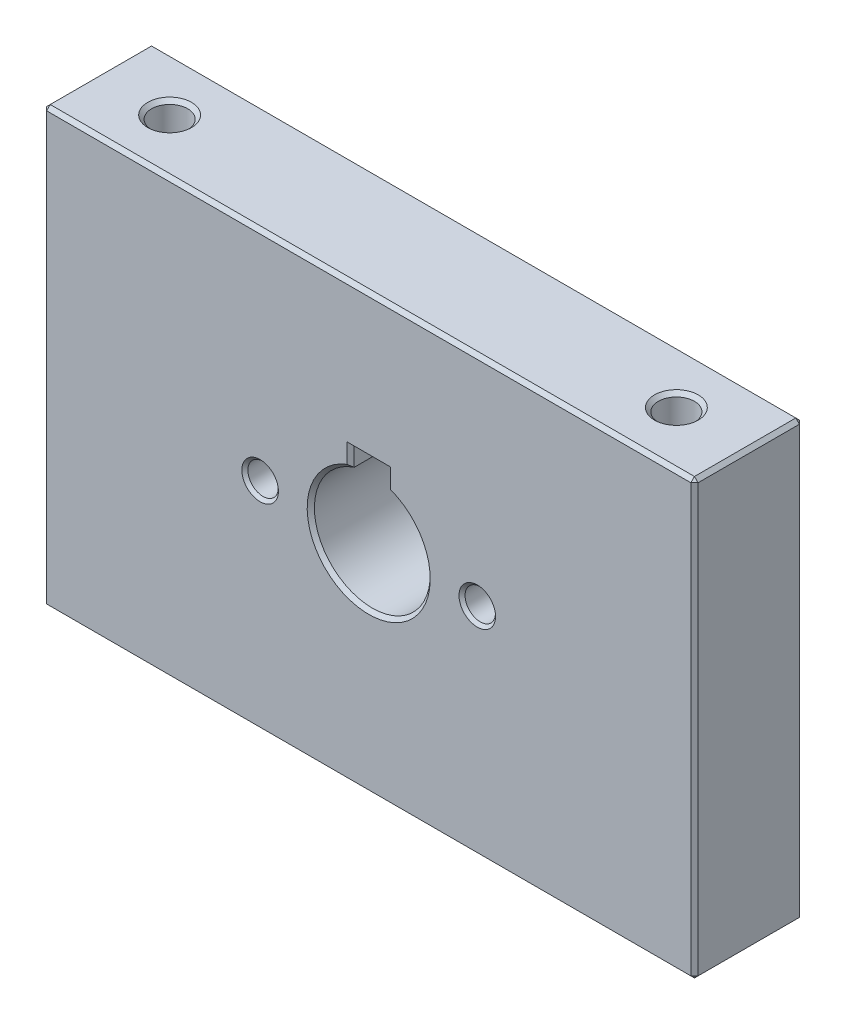
from build123d import *

# Parameters (mm, degrees)
SKETCH_1_W                   = 90
SKETCH_1_H                   = 60
EXTRUDE_1_DEPTH              = 15
SKETCH_3_R                   = 8
CUT_EXTRUDE_1_DEPTH          = 57.124860802
SKETCH_4_W                   = 5
SKETCH_4_H                   = 5.148629024
CUT_EXTRUDE_2_DEPTH          = 20
HOLE_WIZARD_M5_1_D           = 4.2
HOLE_WIZARD_M5_1_DEPTH       = 12.4
HOLE_WIZARD_M5_1_CSINK_D     = 5.05
HOLE_WIZARD_M5_1_CSINK_ANGLE = 92
HOLE_WIZARD_M5_1_TIP         = 1.2618073
SKETCH_8_R                   = 2
CUT_EXTRUDE_4_DEPTH          = 10
HOLE_WIZARD_M6_1_D           = 5
HOLE_WIZARD_M6_1_DEPTH       = 15
HOLE_WIZARD_M6_1_CSINK_D     = 6.05
HOLE_WIZARD_M6_1_CSINK_ANGLE = 92
HOLE_WIZARD_M6_1_TIP         = 1.502151548
HOLE_WIZARD_M6_2_D           = 5
HOLE_WIZARD_M6_2_DEPTH       = 15
HOLE_WIZARD_M6_2_CSINK_D     = 6.05
HOLE_WIZARD_M6_2_CSINK_ANGLE = 92
HOLE_WIZARD_M6_2_TIP         = 1.502151548
CHAMFER_2_SIZE               = 0.5
CHAMFER_3_SIZE               = 0.5


with BuildPart() as part:
    # 草图1 → 凸台-拉伸1 (new body)
    with BuildSketch(Plane.XY):
        Rectangle(SKETCH_1_W, SKETCH_1_H)
    extrude(amount=EXTRUDE_1_DEPTH)

    # 草图3 → 切除-拉伸1 (cut, through all)
    with BuildSketch(Plane.XY.offset(15)):
        Circle(SKETCH_3_R)
    extrude(amount=-CUT_EXTRUDE_1_DEPTH, mode=Mode.SUBTRACT)

    # 草图4 → 切除-拉伸2 (cut)
    with BuildSketch(Plane.XY.offset(15)):
        with Locations((0, 7.574314512)):
            Rectangle(SKETCH_4_W, SKETCH_4_H)
    extrude(amount=-CUT_EXTRUDE_2_DEPTH, mode=Mode.SUBTRACT)

    # M5 螺纹孔1
    with Locations(Plane.XY.offset(15)):
        with Locations((15, 0), (-15, 0)):
            CounterSinkHole(HOLE_WIZARD_M5_1_D / 2, HOLE_WIZARD_M5_1_CSINK_D / 2, depth=HOLE_WIZARD_M5_1_DEPTH, counter_sink_angle=HOLE_WIZARD_M5_1_CSINK_ANGLE)
            with Locations((0, 0, -(HOLE_WIZARD_M5_1_DEPTH + HOLE_WIZARD_M5_1_TIP / 2))):  # 118° drill point
                Cone(0, HOLE_WIZARD_M5_1_D / 2, HOLE_WIZARD_M5_1_TIP, mode=Mode.SUBTRACT)

    # 草图8 → 切除-拉伸4 (cut)
    with BuildSketch(Plane.XZ.offset(30)):
        with Locations(Location((-23, 7.5, 0), (0, 0, 270))):
            Circle(SKETCH_8_R)
        with Locations(Location((23, 7.5, 0), (0, 0, 270))):
            Circle(SKETCH_8_R)
    extrude(amount=-CUT_EXTRUDE_4_DEPTH, mode=Mode.SUBTRACT)

    # M6 螺纹孔1
    with Locations(Plane(origin=(0, 30, 0), x_dir=(1, 0, 0), z_dir=(0, 1, 0))):
        with Locations((-35, -7.5), (35, -7.5)):
            CounterSinkHole(HOLE_WIZARD_M6_1_D / 2, HOLE_WIZARD_M6_1_CSINK_D / 2, depth=HOLE_WIZARD_M6_1_DEPTH, counter_sink_angle=HOLE_WIZARD_M6_1_CSINK_ANGLE)
            with Locations((0, 0, -(HOLE_WIZARD_M6_1_DEPTH + HOLE_WIZARD_M6_1_TIP / 2))):  # 118° drill point
                Cone(0, HOLE_WIZARD_M6_1_D / 2, HOLE_WIZARD_M6_1_TIP, mode=Mode.SUBTRACT)

    # M6 螺纹孔2
    with Locations(Plane(origin=(0, -30, 0), x_dir=(-1, 0, 0), z_dir=(0, -1, 0))):
        with Locations((35, -7.5), (-35, -7.5)):
            CounterSinkHole(HOLE_WIZARD_M6_2_D / 2, HOLE_WIZARD_M6_2_CSINK_D / 2, depth=HOLE_WIZARD_M6_2_DEPTH, counter_sink_angle=HOLE_WIZARD_M6_2_CSINK_ANGLE)
            with Locations((0, 0, -(HOLE_WIZARD_M6_2_DEPTH + HOLE_WIZARD_M6_2_TIP / 2))):  # 118° drill point
                Cone(0, HOLE_WIZARD_M6_2_D / 2, HOLE_WIZARD_M6_2_TIP, mode=Mode.SUBTRACT)

    # 倒角2
    chamfer_2_edges = [part.edges().sort_by_distance(p)[0] for p in [
        (-45, 0, 15),
        (0, -30, 15),
        (45, 0, 15),
        (0, -30, 0),
        (-45, 0, 0),
        (0, 30, 0),
        (45, 0, 0),
        (0, 30, 15),
        (45, -30, 7.5),
        (-45, -30, 7.5),
        (-45, 30, 7.5),
        (45, 30, 7.5),
    ]]
    chamfer(chamfer_2_edges, length=CHAMFER_2_SIZE)

    # 倒角3
    chamfer_3_edges = [part.edges().sort_by_distance(p)[0] for p in [
        (0, -8, 0),
        (0, -8, 15),
        (0, 10.148629024, 0),
        (-2.5, 8.87398555, 0),
        (2.5, 8.87398555, 0),
        (-2.5, 8.87398555, 15),
        (2.5, 8.87398555, 15),
        (0, 10.148629024, 15),
    ]]
    chamfer(chamfer_3_edges, length=CHAMFER_3_SIZE)


solid = part.part
